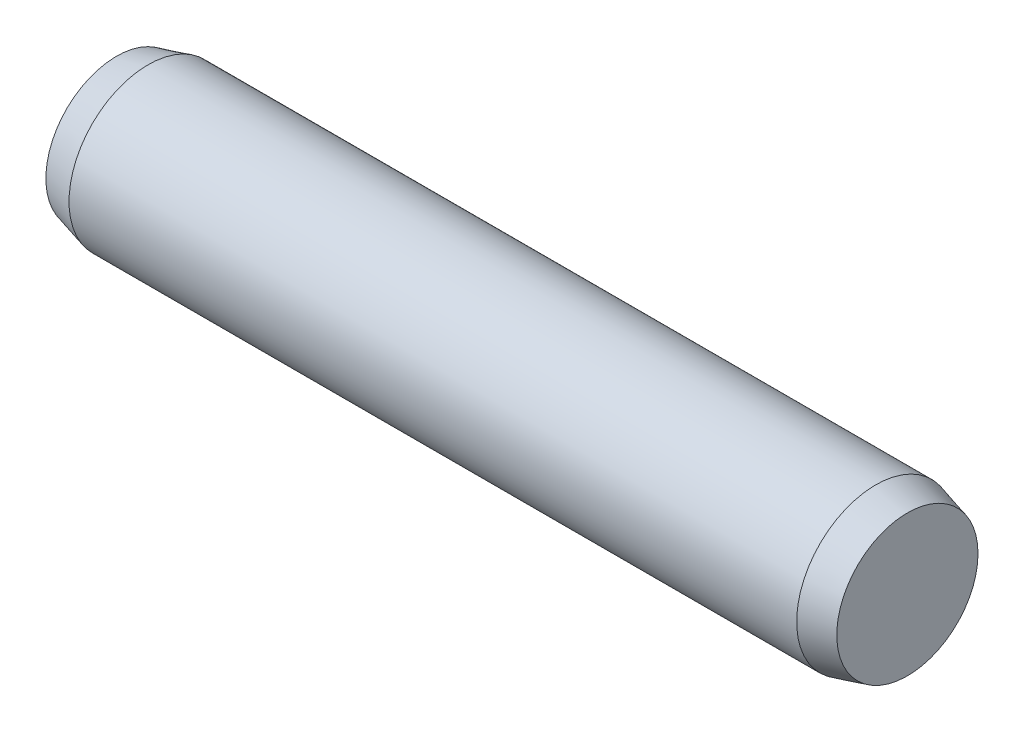
SolidWorks part; units mm, degrees
ref_plane "Front Plane" through (0, 0, 0) normal (0, 0, 1) x (1, 0, 0)
ref_plane "Top Plane" through (0, 0, 0) normal (0, 1, 0) x (1, 0, 0)
ref_plane "Right Plane" through (0, 0, 0) normal (1, 0, 0) x (0, 0, -1)
sketch "Dimensioned Sketch" plane through (0, 0, 0) normal (0, 0, 1) x (1, 0, 0)
  line L0 (0, 0) -> (-0.7681, 0) construction
  line L1 (0, 0) -> (40, 0)
  line L2 (1.6, 4) -> (38.4, 4)
  line L3 (40, 3.5713) -> (40, 0)
  line L4 (38.4, 4) -> (40, 3.5713)
  line L5 (1.6, -4) -> (38.4, -4) construction
  line L6 (1.6, 4) -> (0, 3.5713)
  line L7 (0, 3.5713) -> (0, 0)
  point P13 (20, 4)
  dimension "D1" = 165
  dimension "D2" = 1.6
  dimension "D3" = 165
  dimension "c" = 1.6
  dimension "l" = 40
  dimension "d" = 8
revolve "Base-Revolve" add sketch "Dimensioned Sketch" angle 360 about L0
